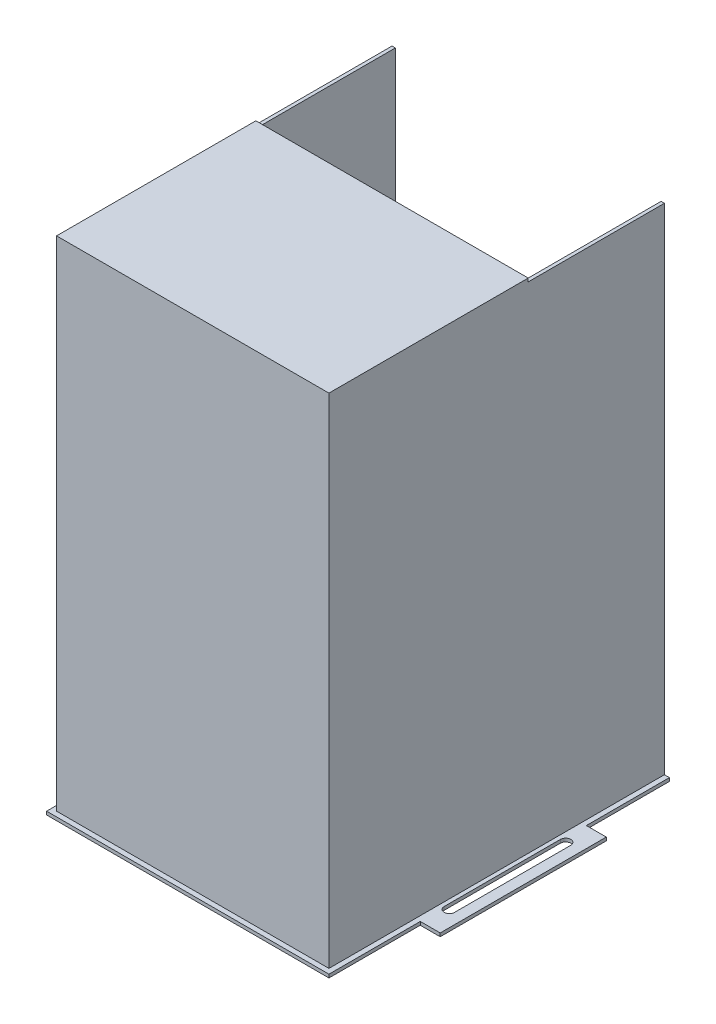
SolidWorks part; units mm, degrees
ref_plane "Front Plane" through (0, 0, 0) normal (0, 0, 1) x (1, 0, 0)
ref_plane "Top Plane" through (0, 0, 0) normal (0, 1, 0) x (1, 0, 0)
ref_plane "Right Plane" through (0, 0, 0) normal (1, 0, 0) x (0, 0, -1)
sketch "Sketch1" plane through (0, 0, 0) normal (0, 1, 0) x (1, 0, 0)
  line L1 (160, 0) -> (160, 200)
  line L2 (0, 0) -> (0, 200)
  line L6 (0, 0) -> (160, 0)
  line L7 (-2, -2) -> (-2, 200)
  line L8 (-2, -2) -> (162, -2)
  line L9 (162, -2) -> (162, 200)
  line L10 (-2, 200) -> (0, 200)
  line L11 (160, 200) -> (162, 200)
  point P12 (160, 0)
  dimension "D1" = 2
  dimension "D2" = 160
  dimension "D3" = 200
  dimension "D4" = 200
extrude "Boss-Extrude1" add sketch "Sketch1" along normal blind 300
sketch "Sketch4" plane through (0, 0, 0) normal (0, -1, 0) x (1, 0, 0)
  line L0 (-2, -200) -> (-2, 2) construction
  line L1 (-2, -50) -> (-17, -50)
  line L2 (-2, -50) -> (-2, -150)
  line L3 (-2, -150) -> (-17, -150)
  line L4 (-17, -50) -> (-17, -150)
  line L5 (162, 2) -> (162, -200) construction
  line L6 (162, -50) -> (177, -50)
  line L7 (162, -50) -> (162, -150)
  line L8 (162, -150) -> (177, -150)
  line L9 (177, -50) -> (177, -150)
  line L10 (162, -200) -> (160, -200) construction
  line L11 (0, -200) -> (-2, -200) construction
  dimension "D1" = 15
  dimension "D2" = 100
  dimension "D3" = 50
  dimension "D4" = 15
  dimension "D5" = 50
  dimension "D6" = 100
extrude "Boss-Extrude3" add sketch "Sketch4" against normal blind 2
sketch "Sketch5" plane through (0, 0, 0) normal (0, -1, 0) x (1, 0, 0)
  line L0 (-7.5, -65) -> (-7.5, -135) construction
  line L1 (-4.4, -65) -> (-4.4, -135)
  line L2 (-10.6, -65) -> (-10.6, -135)
  line L3 (167.5, -65) -> (167.5, -135) construction
  line L4 (170.6, -65) -> (170.6, -135)
  line L5 (164.4, -65) -> (164.4, -135)
  line L6 (177, -150) -> (177, -50) construction
  line L7 (162, -150) -> (177, -150) construction
  line L8 (-17, -50) -> (-17, -150) construction
  line L9 (-17, -150) -> (-2, -150) construction
  arc A0 (-4.4, -65) -> (-10.6, -65) centre (-7.5, -65) ccw
  arc A1 (-10.6, -135) -> (-4.4, -135) centre (-7.5, -135) ccw
  arc A2 (170.6, -65) -> (164.4, -65) centre (167.5, -65) ccw
  arc A3 (164.4, -135) -> (170.6, -135) centre (167.5, -135) ccw
  point P2 (-7.5, -100)
  point P7 (167.5, -100)
  dimension "D1" = 3.1
  dimension "D5" = 3.1
  dimension "D2" = 9.5
  dimension "D3" = 70
  dimension "D4" = 50
  dimension "D6" = 70
  dimension "D7" = 9.5
  dimension "D8" = 50
  dimension "D9" = 175
extrude "Cut-Extrude2" cut sketch "Sketch5" against normal through all both and the other way through all
sketch "Sketch6" plane through (0, 300, 0) normal (0, 1, 0) x (1, 0, 0)
  line L6 (162, -2) -> (162, 200) construction
  line L7 (-2, -2) -> (162, -2)
  line L8 (-2, -2) -> (-2, 118)
  line L9 (-2, 118) -> (162, 118)
  line L10 (162, -2) -> (162, 118)
  dimension "D1" = 120
extrude "Boss-Extrude4" add sketch "Sketch6" along normal blind 2
sketch "Sketch7" plane through (0, 0, 0) normal (0, -1, 0) x (1, 0, 0)
  line L0 (-2, -200) -> (-2, 2)
  line L1 (-2, 2) -> (162, 2)
  line L2 (162, 2) -> (162, -200)
  line L3 (-5, -200) -> (-5, -137.9668)
  line L4 (-5, 5) -> (165, 5)
  line L5 (165, 5) -> (165, -56.3047)
  line L6 (-5, -200) -> (-2, -200)
  line L7 (162, -200) -> (165, -200)
  line L8 (165, -137.9668) -> (163.3873, -137.9668)
  line L9 (163.3873, -137.9668) -> (163.3873, -56.3047)
  line L10 (163.3873, -56.3047) -> (165, -56.3047)
  line L11 (-5, -59.2537) -> (-3.5, -59.2537)
  line L12 (-3.5, -59.2537) -> (-3.5, -137.9668)
  line L13 (-3.5, -137.9668) -> (-5, -137.9668)
  line L14 (-5, -59.2537) -> (-5, 5)
  line L15 (-5, -200) -> (-5, 5) construction
  line L16 (165, -137.9668) -> (165, -200)
  line L17 (165, 5) -> (165, -200) construction
  dimension "D1" = 3
extrude "Boss-Extrude5" add sketch "Sketch7" against normal blind 2
